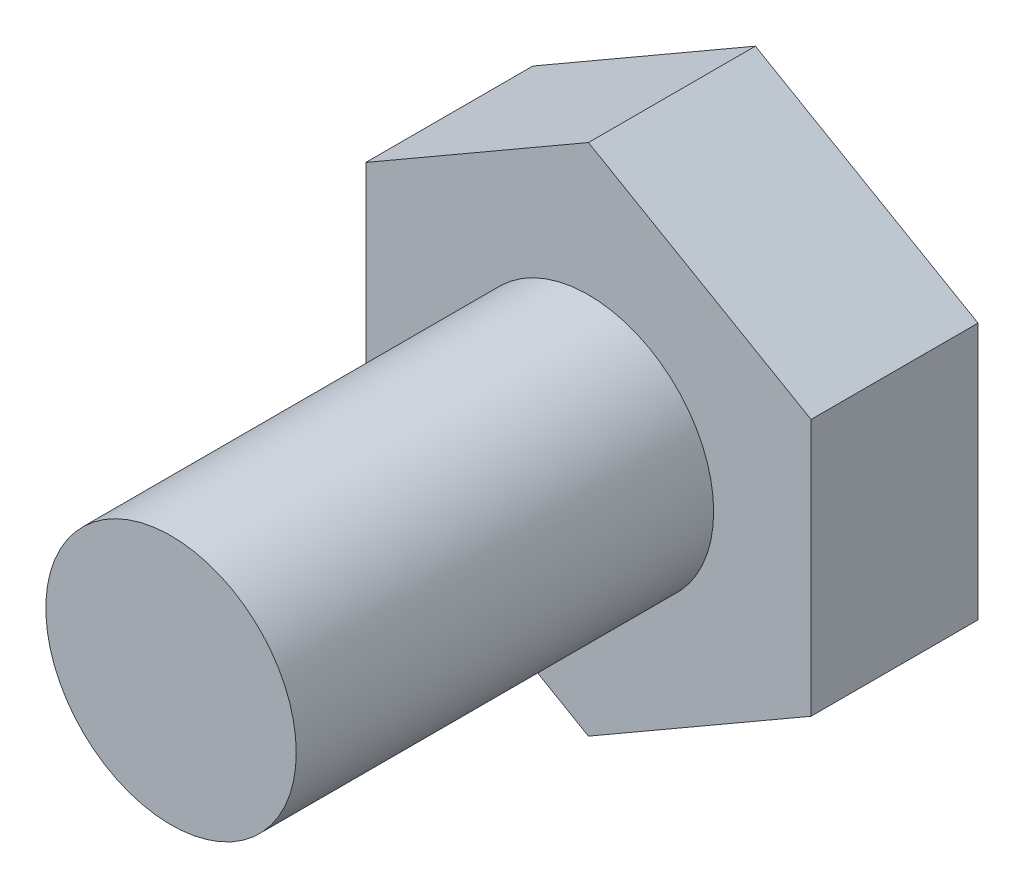
from build123d import *

# Parameters (mm, degrees)
BOSS_EXTRUDE2_DEPTH = 6
SKETCH3_R           = 4.5
BOSS_EXTRUDE3_DEPTH = 15


with BuildPart() as part:
    # Sketch2 → Boss-Extrude2 (new body)
    with BuildSketch(Plane.XY):
        Polygon((0, 9.237604307), (-8, 4.618802154), (-8, -4.618802154), (0, -9.237604307), (8, -4.618802154), (8, 4.618802154), align=None)
    extrude(amount=BOSS_EXTRUDE2_DEPTH)

    # Sketch3 → Boss-Extrude3 (add)
    with BuildSketch(Plane.XY.offset(6)):
        Circle(SKETCH3_R)
    extrude(amount=BOSS_EXTRUDE3_DEPTH)


solid = part.part
